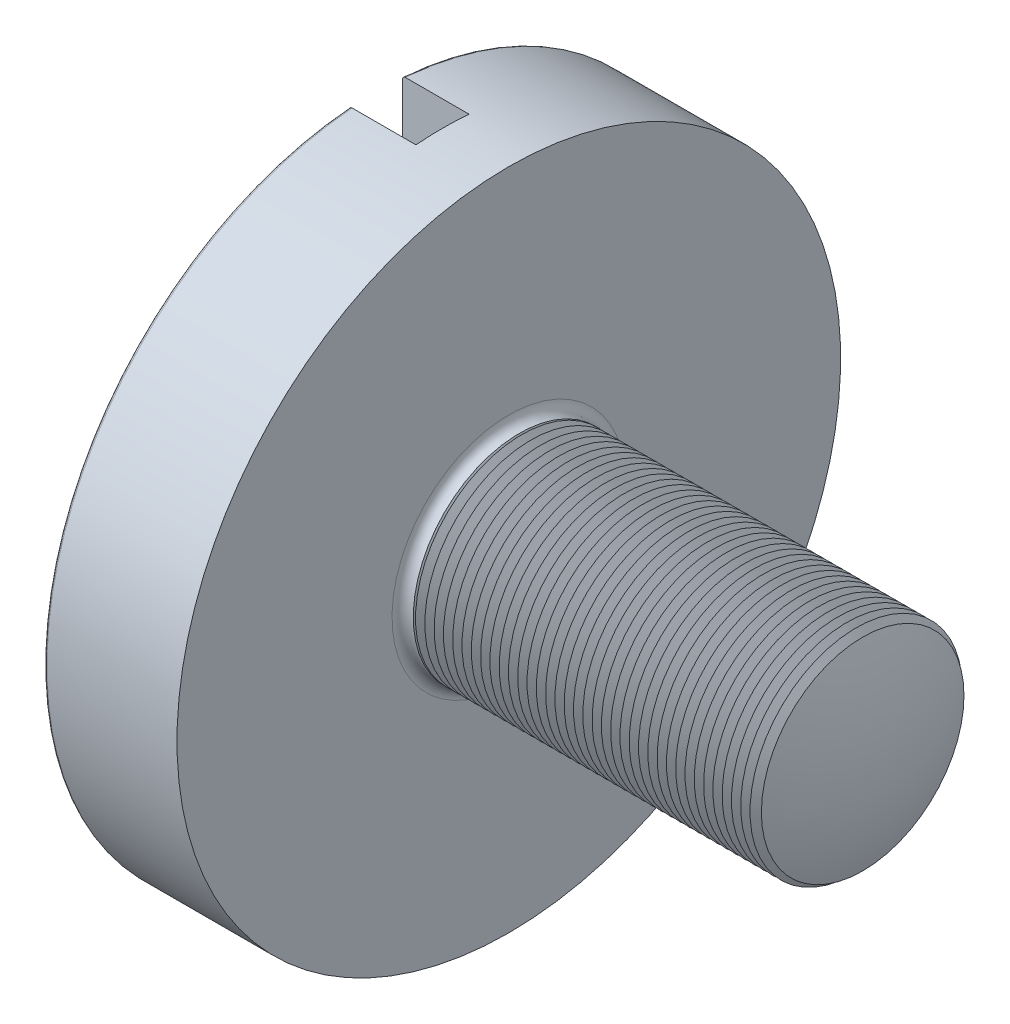
from build123d import *

# Parameters (mm, degrees)
CUT_EXTRUDE_START      = -2.5
CUT_EXTRUDE_1_DEPTH    = 2.5
FILLET_1_R             = 0.1
PATTERN_LINEAR_1_COUNT = 39
PATTERN_LINEAR_1_PITCH = 0.35


with BuildPart() as part:
    # 草图1 → Revolve 584 (revolve)
    with BuildSketch(Plane.XY, mode=Mode.PRIVATE) as revolve_584_sk:
        with BuildLine():
            Line((0, 0), (0, 12.5))
            Line((0, 12.5), (5, 12.5))
            Line((5, 12.5), (5, 4.4))
            ThreePointArc((5, 4.4), (5.117157288, 4.117157288), (5.4, 4))
            Line((5.4, 4), (18.261357464, 4))
            ThreePointArc((18.261357464, 4), (18.813791436, 2.033813708), (19, 0))
            Line((19, 0), (0, 0))
        make_face()
    revolve(revolve_584_sk.sketch.rotate(Axis((0, 0, 0), (1, 0, 0)), 180), axis=Axis((0, 0, 0), (1, 0, 0)))

    # 草图2 → 切除-拉伸1 (cut)
    with BuildSketch(Plane.ZY.offset(CUT_EXTRUDE_START)):
        with BuildLine():
            Line((1, 12.459935794), (1, -12.459935794))
            ThreePointArc((1, -12.459935794), (0, -12.5), (-1, -12.459935794))
            Line((-1, -12.459935794), (-1, 12.459935794))
            ThreePointArc((-1, 12.459935794), (0, 12.5), (1, 12.459935794))
        make_face()
    extrude(amount=CUT_EXTRUDE_1_DEPTH, mode=Mode.SUBTRACT)

    # 圆角1
    fillet_1_edges = [part.edges().sort_by_distance(p)[0] for p in [
        (0, 0, -12.5),
        (0, 0, 12.5),
    ]]
    fillet(fillet_1_edges, radius=FILLET_1_R)

    # 草图3 → 切除-旋转1 (revolve, cut)
    with BuildSketch(Plane.XY, mode=Mode.PRIVATE) as cut_revolve_1_sk:
        Polygon((18.086362598, 4), (18.436352331, 4), (18.261357464, 3.6969), align=None)
    cut_revolve_1 = revolve(cut_revolve_1_sk.sketch.rotate(Axis((0, 0, 0), (-1, 0, 0)), 90), axis=Axis((0, 0, 0), (-1, 0, 0)), mode=Mode.SUBTRACT)

    # 阵列(线性)1: 切除-旋转1 ×39
    with Locations(*[(-i * PATTERN_LINEAR_1_PITCH, 0, 0) for i in range(1, PATTERN_LINEAR_1_COUNT)]):
        add(cut_revolve_1, mode=Mode.SUBTRACT)


solid = part.part
